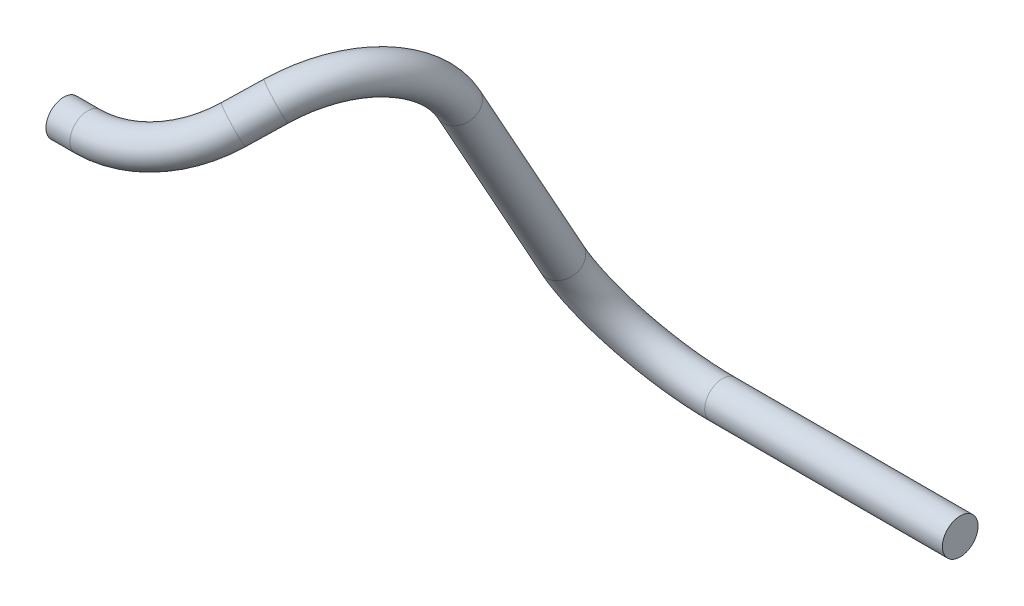
from build123d import *

# Parameters (mm, degrees)
SKETCH2_R = 2


with BuildPart() as part:
    # Sweep1: sweep along a curve in space
    with BuildLine() as sweep1_path:
        Line((-19.39826571, 55.978701071, 2.254926967), (-16.715694993, 55.978701071, 2.254926967))
        ThreePointArc((-6.047634181, 59.123559398, -3.439623567), (-10.468184265, 56.826927396, 0.719001604), (-16.715694993, 55.978701071, 2.254926967))
        Line((-6.047634181, 59.123559398, -3.439623567), (-4.269895959, 60.792120921, -6.460970453))
        ThreePointArc((0.98288182, 55.507835041, -21.708417726), (-0.455385422, 61.380619924, -14.795022607), (-4.269895959, 60.792120921, -6.460970453))
        Line((0.98288182, 55.507835041, -21.708417726), (0.488315483, 34.167885645, -33.784564331))
        ThreePointArc((12.48587526, 23.513552475, -39.813786189), (3.915464358, 26.647289087, -38.040423843), (0.488315483, 34.167885645, -33.784564331))
        Line((12.48587526, 23.513552475, -39.813786189), (39.17173429, 23.513552475, -39.813786189))
    # Sketch2 → Sweep1 (sweep)
    with BuildSketch(Plane(origin=(-19.39826571, 0, 0), x_dir=(0, 0, -1), z_dir=(1, 0, 0))):
        with Locations((-2.254926967, 55.978701071)):
            Circle(SKETCH2_R)
    sweep(path=sweep1_path.line)


solid = part.part
